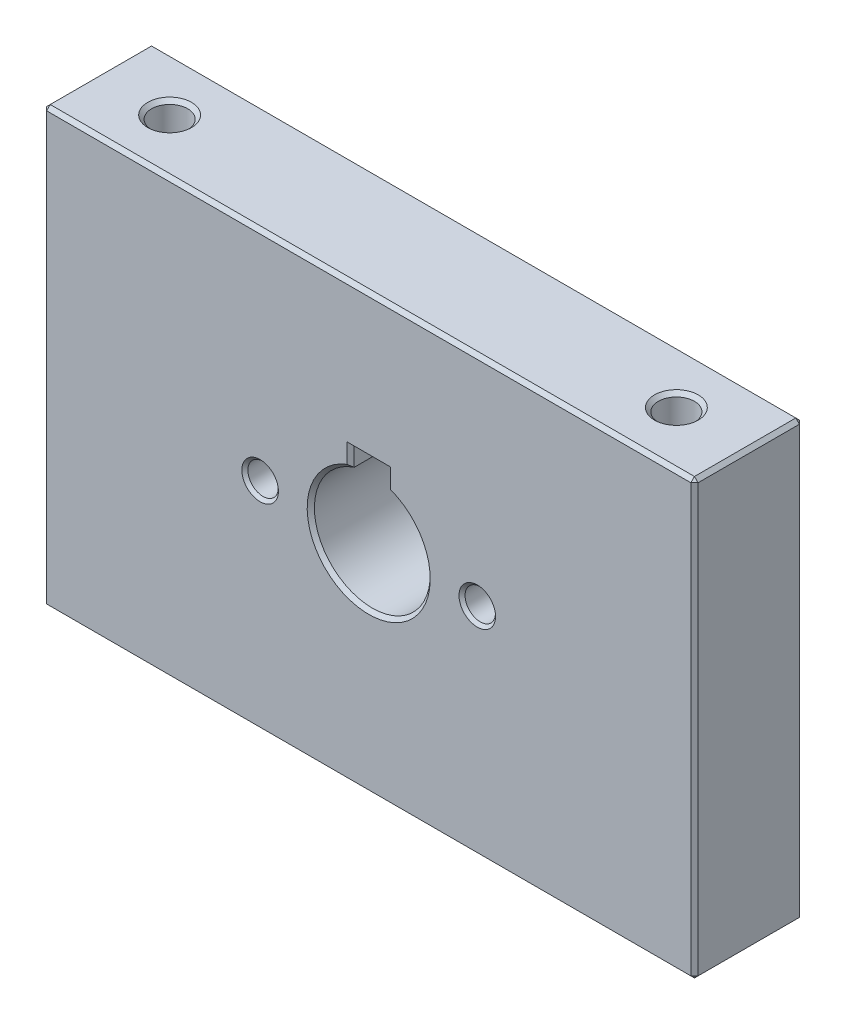
SolidWorks part; units mm, degrees
material "45#"
ref_plane "前视基准面" through (0, 0, 0) normal (0, 0, 1) x (1, 0, 0)
ref_plane "上视基准面" through (0, 0, 0) normal (0, 1, 0) x (1, 0, 0)
ref_plane "右视基准面" through (0, 0, 0) normal (1, 0, 0) x (0, 0, -1)
sketch "草图1" plane through (0, 0, 0) normal (0, 0, 1) x (1, 0, 0)
  line L1 (-45, 30) -> (45, 30)
  line L2 (-45, 30) -> (-45, -30)
  line L3 (-45, -30) -> (45, -30)
  line L4 (45, 30) -> (45, -30)
  line L5 (-45, 30) -> (45, -30) construction
  line L6 (-45, -30) -> (45, 30) construction
  point P0 (0, 0)
  dimension "D1" = 60
  dimension "D2" = 90
extrude "凸台-拉伸1" add sketch "草图1" along normal blind 15
sketch "草图3" plane through (0, 0, 15) normal (0, 0, 1) x (1, 0, 0)
  circle A0 centre (0, 0) radius 8
  dimension "D1" = 16
extrude "切除-拉伸1" cut sketch "草图3" against normal through all
sketch "草图4" plane through (0, 0, 15) normal (0, 0, 1) x (1, 0, 0)
  line L1 (-2.5, 10.1486) -> (2.5, 10.1486)
  line L2 (-2.5, 10.1486) -> (-2.5, 5)
  line L3 (-2.5, 5) -> (2.5, 5)
  line L4 (2.5, 10.1486) -> (2.5, 5)
  dimension "D1" = 5
  dimension "D2" = 2.5
  dimension "D3" = 5
extrude "切除-拉伸2" cut sketch "草图4" against normal blind 20
hole_wizard "M5 螺纹孔1" positions "草图5" profile "草图6" tap size "M5" standard "AS"
sketch "草图5" plane through (0, 0, 15) normal (0, 0, 1) x (1, 0, 0)
  point P3 (15, 0)
  point P6 (-15, 0)
sketch "草图6" plane through (15, 0, 15) normal (1, 0, 0) x (0, -1, 0)
  line L0 (0, 0) -> (0, 13.6618)
  line L1 (0, 13.6618) -> (2.1, 12.4)
  line L2 (2.1, 12.4) -> (2.1, 0.4104)
  line L3 (2.1, 0.4104) -> (2.525, 0)
  line L5 (2.525, 0) -> (0, 0)
  line L6 (-2.1, 0.4104) -> (-2.525, 0) construction
  line L10 (0, 13.6618) -> (-2.1, 12.4) construction
  line L11 (0, -6.35) -> (0, 107.95) construction
  dimension "螺纹孔钻头直径" = 4.2
  dimension "螺纹孔钻头深度" = 12.4
  dimension "近端锥形沉头孔直径" = 5.05
  dimension "近端锥形沉头孔角度" = 92
  dimension "导头角度" = 118
cosmetic thread "孔螺蚊线1" parameters "D1"=10, "D2"=5
cosmetic thread "孔螺蚊线2" parameters "D1"=10, "D2"=5
sketch "草图8" plane through (0, -30, 0) normal (0, -1, 0) x (1, 0, 0)
  circle A0 centre (-23, 7.5) radius 2
  circle A1 centre (23, 7.5) radius 2
  dimension "D1" = 4
  dimension "D2" = 4
extrude "切除-拉伸4" cut sketch "草图8" against normal blind 10
hole_wizard "M6 螺纹孔1" positions "草图9" profile "草图11" tap size "M6" standard "AS"
sketch "草图9" plane through (0, 30, 0) normal (0, 1, 0) x (1, 0, 0)
  point P2 (-35, -7.5)
  point P5 (35, -7.5)
sketch "草图11" plane through (-35, 30, 7.5) normal (1, 0, 0) x (0, 0, 1)
  line L0 (0, 0) -> (0, 16.5022)
  line L1 (0, 16.5022) -> (2.5, 15)
  line L2 (2.5, 15) -> (2.5, 0.507)
  line L3 (2.5, 0.507) -> (3.025, 0)
  line L5 (3.025, 0) -> (0, 0)
  line L6 (-2.5, 0.507) -> (-3.025, 0) construction
  line L10 (0, 16.5022) -> (-2.5, 15) construction
  line L11 (0, -6.35) -> (0, 107.95) construction
  dimension "螺纹孔钻头直径" = 5
  dimension "螺纹孔钻头深度" = 15
  dimension "近端锥形沉头孔直径" = 6.05
  dimension "近端锥形沉头孔角度" = 92
  dimension "导头角度" = 118
cosmetic thread "孔螺蚊线3" parameters "D1"=12, "D2"=6
cosmetic thread "孔螺蚊线4" parameters "D1"=12, "D2"=6
hole_wizard "M6 螺纹孔2" positions "草图12" profile "草图13" tap size "M6" standard "AS"
sketch "草图12" plane through (0, -30, 0) normal (0, -1, 0) x (-1, 0, 0)
  point P0 (35, -7.5)
  point P3 (-35, -7.5)
sketch "草图13" plane through (-35, -30, 7.5) normal (1, 0, 0) x (0, 0, -1)
  line L0 (0, 0) -> (0, 16.5022)
  line L1 (0, 16.5022) -> (2.5, 15)
  line L2 (2.5, 15) -> (2.5, 0.507)
  line L3 (2.5, 0.507) -> (3.025, 0)
  line L5 (3.025, 0) -> (0, 0)
  line L6 (-2.5, 0.507) -> (-3.025, 0) construction
  line L10 (0, 16.5022) -> (-2.5, 15) construction
  line L11 (0, -6.35) -> (0, 107.95) construction
  dimension "螺纹孔钻头直径" = 5
  dimension "螺纹孔钻头深度" = 15
  dimension "近端锥形沉头孔直径" = 6.05
  dimension "近端锥形沉头孔角度" = 92
  dimension "导头角度" = 118
cosmetic thread "孔螺蚊线5" parameters "D1"=12, "D2"=6
cosmetic thread "孔螺蚊线6" parameters "D1"=12, "D2"=6
chamfer "倒角2" distance 0.5 angle 45 12 edges at (45, -30, 7.5) (45, 0, 15) (45, 30, 7.5) (45, 0, 0) (-45, 30, 7.5) (0, 30, 15) (-45, 0, 15) (0, -30, 15) (-45, -30, 7.5) (0, 30, 0) (-45, 0, 0) (0, -30, 0)
chamfer "倒角3" distance 0.5 angle 45 8 edges at (0, -8, 0) (-2.5, 8.874, 0) (0, 10.1486, 0) (2.5, 8.874, 0) (2.5, 8.874, 15) (0, 10.1486, 15) (-2.5, 8.874, 15) (0, -8, 15)
